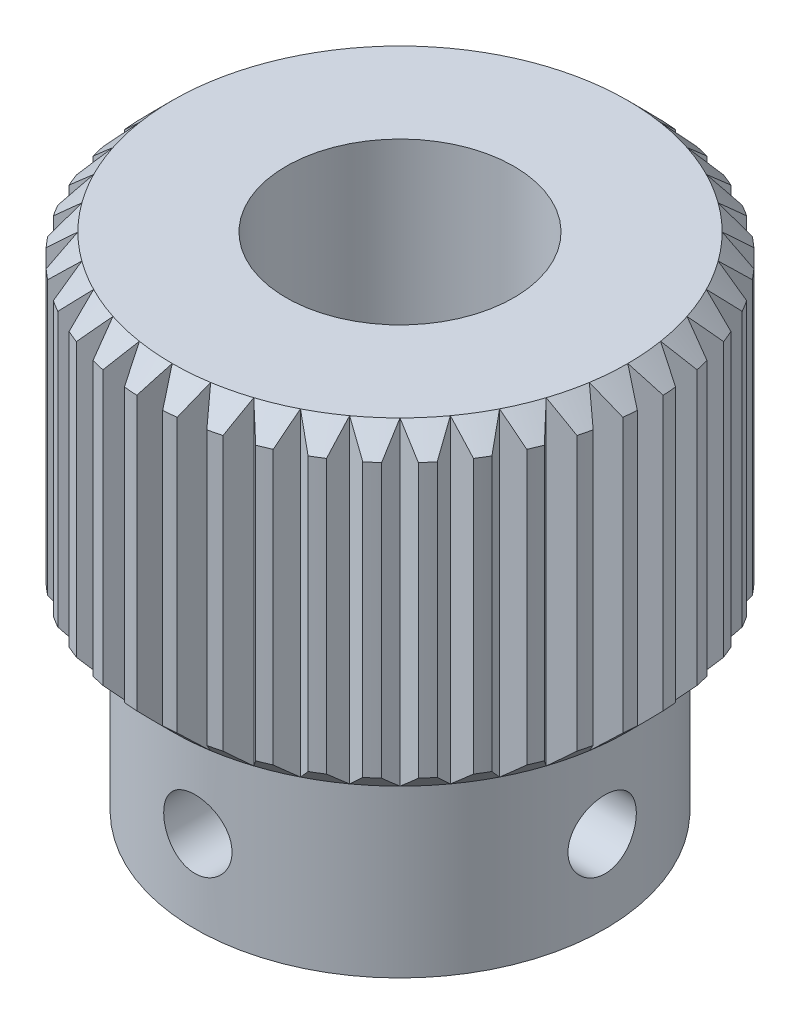
SolidWorks part; units mm, degrees
material "Brass"
ref_plane "Front Plane" through (0, 0, 0) normal (0, 0, 1) x (1, 0, 0)
ref_plane "Top Plane" through (0, 0, 0) normal (0, 1, 0) x (1, 0, 0)
ref_plane "Right Plane" through (0, 0, 0) normal (1, 0, 0) x (0, 0, -1)
sketch "Sketch1" plane through (0, 0, 0) normal (0, 0, 1) x (1, 0, 0)
  line L0 (0, 0) -> (0, 11) construction
  line L1 (2.5, 0) -> (2.5, 11)
  line L2 (2.5, 11) -> (5, 11)
  line L3 (5.5, 10.5) -> (5.5, 4.5)
  line L4 (5, 4) -> (4.5, 4)
  line L5 (4.5, 4) -> (4.5, 0)
  line L6 (4.5, 0) -> (2.5, 0)
  line L7 (5, 11) -> (5.5, 10.5)
  line L8 (5.5, 4.5) -> (5, 4)
  point P5 (5.5, 11)
  point P7 (5.5, 4)
  dimension "D1" = 11
  dimension "D2" = 11
  dimension "D3" = 5
  dimension "D4" = 9
  dimension "D5" = 7
  dimension "D6" = 0.5
  dimension "D7" = 45
  dimension "D8" = 0.5
  dimension "D9" = 45
revolve "Revolve1" add sketch "Sketch1" angle 360 about L0
sketch "Sketch2" plane through (0, 11, 0) normal (0, 1, 0) x (1, 0, 0)
  line L1 (0.433, 5.75) -> (-0.433, 5.75)
  line L2 (-0.433, 5.75) -> (0, 5)
  line L3 (0, 5) -> (0.433, 5.75)
  circle A0 centre (0, 5.5) radius 0.25 construction
  dimension "D1" = 0.5
  dimension "D2" = 5.5
extrude "Cut-Extrude1" cut sketch "Sketch2" against normal through all
pattern_circular "CirPattern1" count 40 over 360 about axis through (0, 0, 0) along (0, 1, 0) of "Cut-Extrude1"
sketch "Sketch3" plane through (0, 0, 0) normal (0, 0, 1) x (1, 0, 0)
  circle A0 centre (0, 1.8044) radius 0.75
  dimension "D1" = 1.5
  dimension "D2" = 1.8044
extrude "Cut-Extrude2" cut sketch "Sketch3" along normal blind 10
sketch "Sketch4" plane through (0, 0, 0) normal (1, 0, 0) x (0, 0, -1)
  circle A0 centre (0, 1.8) radius 0.75
  dimension "D1" = 1.8
  dimension "D2" = 1.5
extrude "Cut-Extrude3" cut sketch "Sketch4" along normal blind 10
